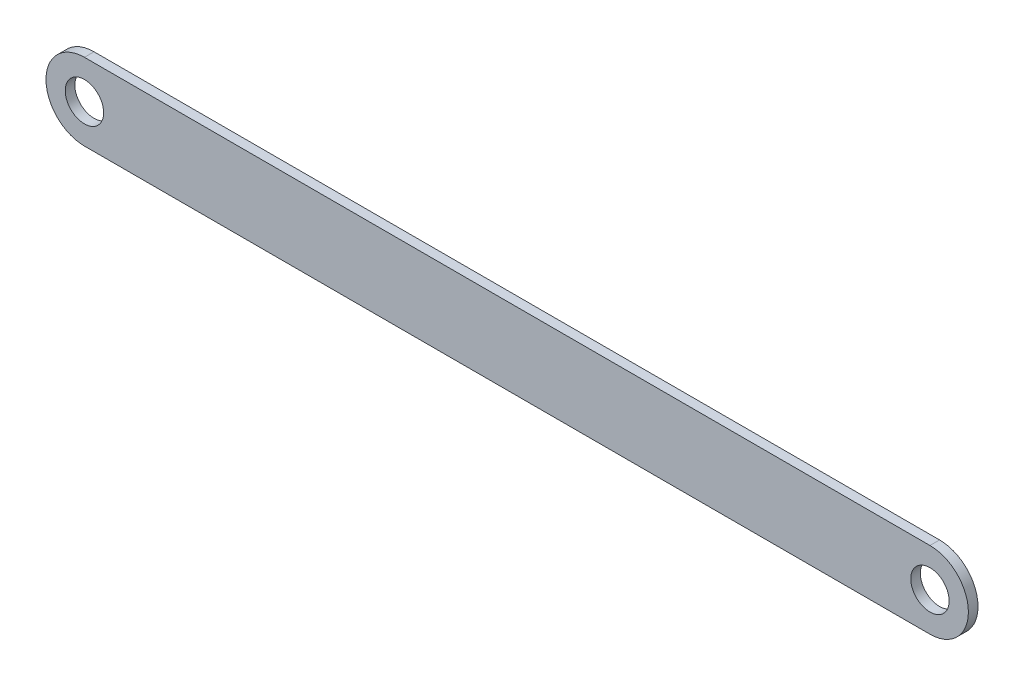
from build123d import *

# Parameters (mm, degrees)
SKETCH1_R           = 5
BOSS_EXTRUDE1_DEPTH = 2.5


with BuildPart() as part:
    # Sketch1 → Boss-Extrude1 (new body)
    with BuildSketch(Plane.XY):
        with BuildLine():
            Line((-110, 10), (110, 10))
            ThreePointArc((110, 10), (120, 0), (110, -10))
            Line((110, -10), (-110, -10))
            ThreePointArc((-110, -10), (-120, 0), (-110, 10))
        make_face()
        with Locations((-110, 0)):
            Circle(SKETCH1_R, mode=Mode.SUBTRACT)
        with Locations((110, 0)):
            Circle(SKETCH1_R, mode=Mode.SUBTRACT)
    extrude(amount=BOSS_EXTRUDE1_DEPTH)


solid = part.part
